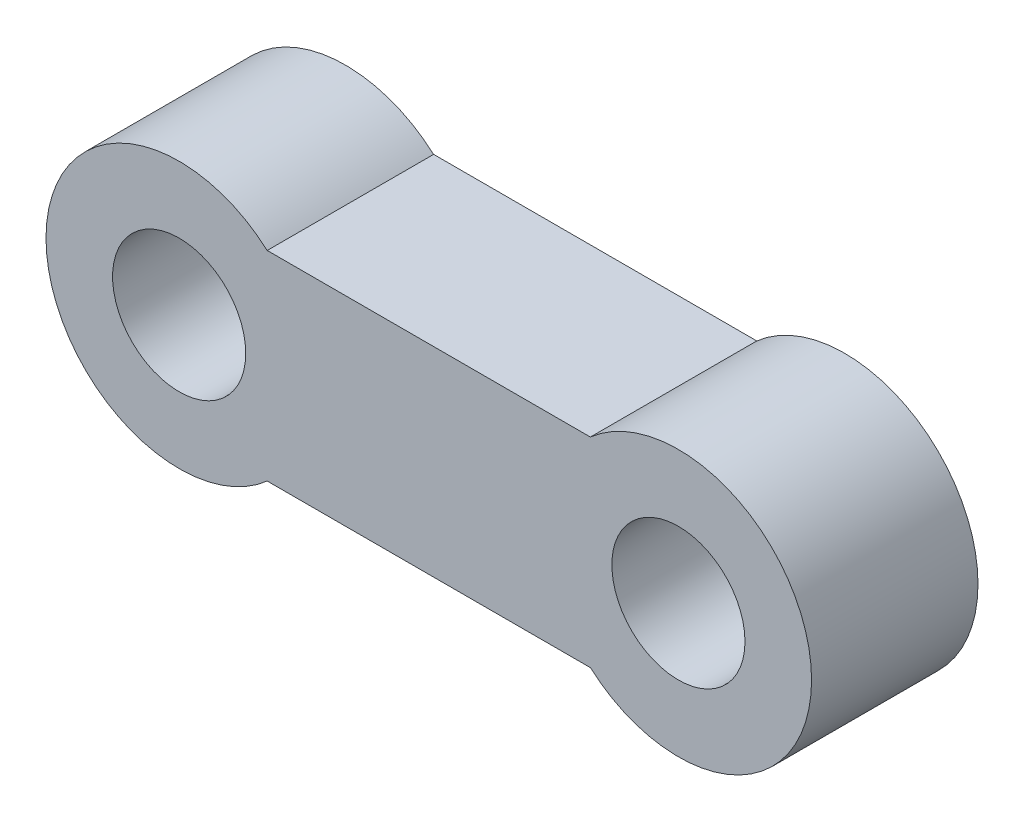
SolidWorks part; units mm, degrees
ref_plane "Front Plane" through (0, 0, 0) normal (0, 0, 1) x (1, 0, 0)
ref_plane "Top Plane" through (0, 0, 0) normal (0, 1, 0) x (1, 0, 0)
ref_plane "Right Plane" through (0, 0, 0) normal (1, 0, 0) x (0, 0, -1)
sketch "Sketch1" plane through (0, 0, 0) normal (0, 0, 1) x (1, 0, 0)
  line L0 (5.2915, -6) -> (24.7085, -6)
  line L1 (5.2915, 6) -> (24.7085, 6)
  line L2 (0, 0) -> (30, 0) construction
  circle A0 centre (0, 0) radius 4
  arc A1 (5.2915, 6) -> (5.2915, -6) centre (0, 0) ccw
  circle A2 centre (30, 0) radius 4
  arc A3 (24.7085, -6) -> (24.7085, 6) centre (30, 0) ccw
  dimension "D1" = 30
  dimension "D2" = 8
  dimension "D3" = 8
  dimension "D4" = 16
  dimension "D5" = 16
  dimension "D6" = 12
  dimension "D7" = 6
extrude "Boss-Extrude1" add sketch "Sketch1" along normal blind 10
